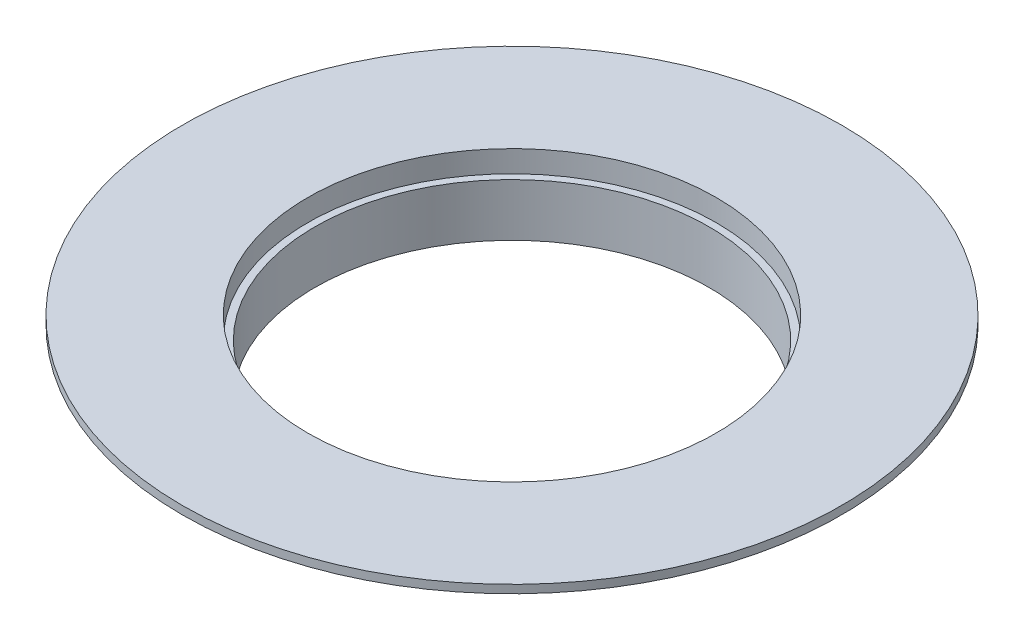
SolidWorks part; units mm, degrees
ref_plane "Front Plane" through (0, 0, 0) normal (0, 0, 1) x (1, 0, 0)
ref_plane "Top Plane" through (0, 0, 0) normal (0, 1, 0) x (1, 0, 0)
ref_plane "Right Plane" through (0, 0, 0) normal (1, 0, 0) x (0, 0, -1)
sketch "Sketch1" plane through (0, 0, 0) normal (0, 0, 1) x (1, 0, 0)
  line L0 (0, 0) -> (0, -32.96) construction
  line L1 (102, 158) -> (65.583, 158)
  line L2 (102, 158) -> (-102, 158) construction
  line L3 (86.2487, 158) -> (-86.2487, 158) construction
  line L4 (65.583, 158) -> (65.583, 151.5)
  line L5 (-68.9957, 151.5) -> (68.9957, 151.5) construction
  line L6 (65.583, 151.5) -> (63.9957, 151.5)
  line L7 (63.9957, 151.5) -> (-63.9957, 151.5) construction
  line L8 (63.9957, 151.5) -> (63.9957, 137.5)
  line L9 (-63.9957, 137.5) -> (63.9957, 137.5) construction
  line L10 (63.9957, 137.5) -> (60.9957, 137.5)
  line L11 (60.9957, 137.5) -> (60.9957, 153.779)
  line L12 (60.9957, 153.779) -> (63.1935, 153.779)
  line L13 (63.1935, 153.779) -> (63.1935, 160.5319)
  line L14 (63.1935, 160.5319) -> (102, 160.5319)
  line L15 (102, 160.5319) -> (102, 158)
revolve "Revolve1" add sketch "Sketch1" angle 360 about L0
